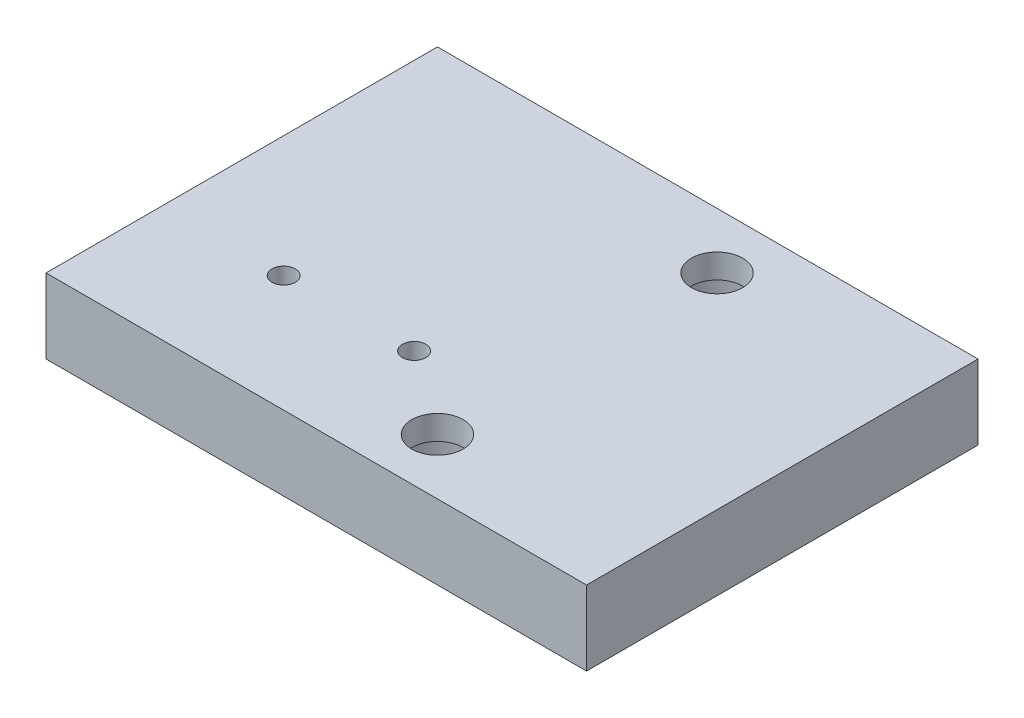
from build123d import *

# Parameters (mm, degrees)
SKETCH_1_W                   = 58
SKETCH_1_H                   = 42
EXTRUDE_1_DEPTH              = 4
HOLE_WIZARD_M5_1_D           = 5.5
HOLE_WIZARD_M5_1_CBORE_D     = 10
HOLE_WIZARD_M5_1_CBORE_DEPTH = 5.4
HOLE_WIZARD_M4_1_D           = 3.3
HOLE_WIZARD_M4_1_DEPTH       = 10.1
HOLE_WIZARD_M4_1_TIP         = 0.991420021
HOLE_WIZARD_M3_1_D           = 2.5


with BuildPart() as part:
    # 草图1 → 凸台-拉伸1 (new, symmetric)
    with BuildSketch(Plane(origin=(0, 0, 0), x_dir=(1, 0, 0), z_dir=(0, 1, 0))):
        Rectangle(SKETCH_1_W, SKETCH_1_H)
    extrude(amount=EXTRUDE_1_DEPTH, both=True)

    # M5 六角凹头螺钉的柱形沉头孔1 (through all)
    with Locations(Plane(origin=(0, -4, 0), x_dir=(-1, 0, 0), z_dir=(0, -1, 0))):
        with Locations((-7, 15), (-7, -15)):
            CounterBoreHole(HOLE_WIZARD_M5_1_D / 2, HOLE_WIZARD_M5_1_CBORE_D / 2, HOLE_WIZARD_M5_1_CBORE_DEPTH)

    # M4 螺纹孔1
    with Locations(Plane.ZY.offset(29)):
        with Locations((-11, 0), (11, 0)):
            Hole(HOLE_WIZARD_M4_1_D / 2, depth=HOLE_WIZARD_M4_1_DEPTH)
            with Locations((0, 0, -(HOLE_WIZARD_M4_1_DEPTH + HOLE_WIZARD_M4_1_TIP / 2))):  # 118° drill point
                Cone(0, HOLE_WIZARD_M4_1_D / 2, HOLE_WIZARD_M4_1_TIP, mode=Mode.SUBTRACT)

    # M3 螺纹孔1 (through all)
    with Locations(Plane(origin=(0, -4, 0), x_dir=(-1, 0, 0), z_dir=(0, -1, 0))):
        with Locations((16, -8.5), (2, -8.5)):
            Hole(HOLE_WIZARD_M3_1_D / 2)


solid = part.part
